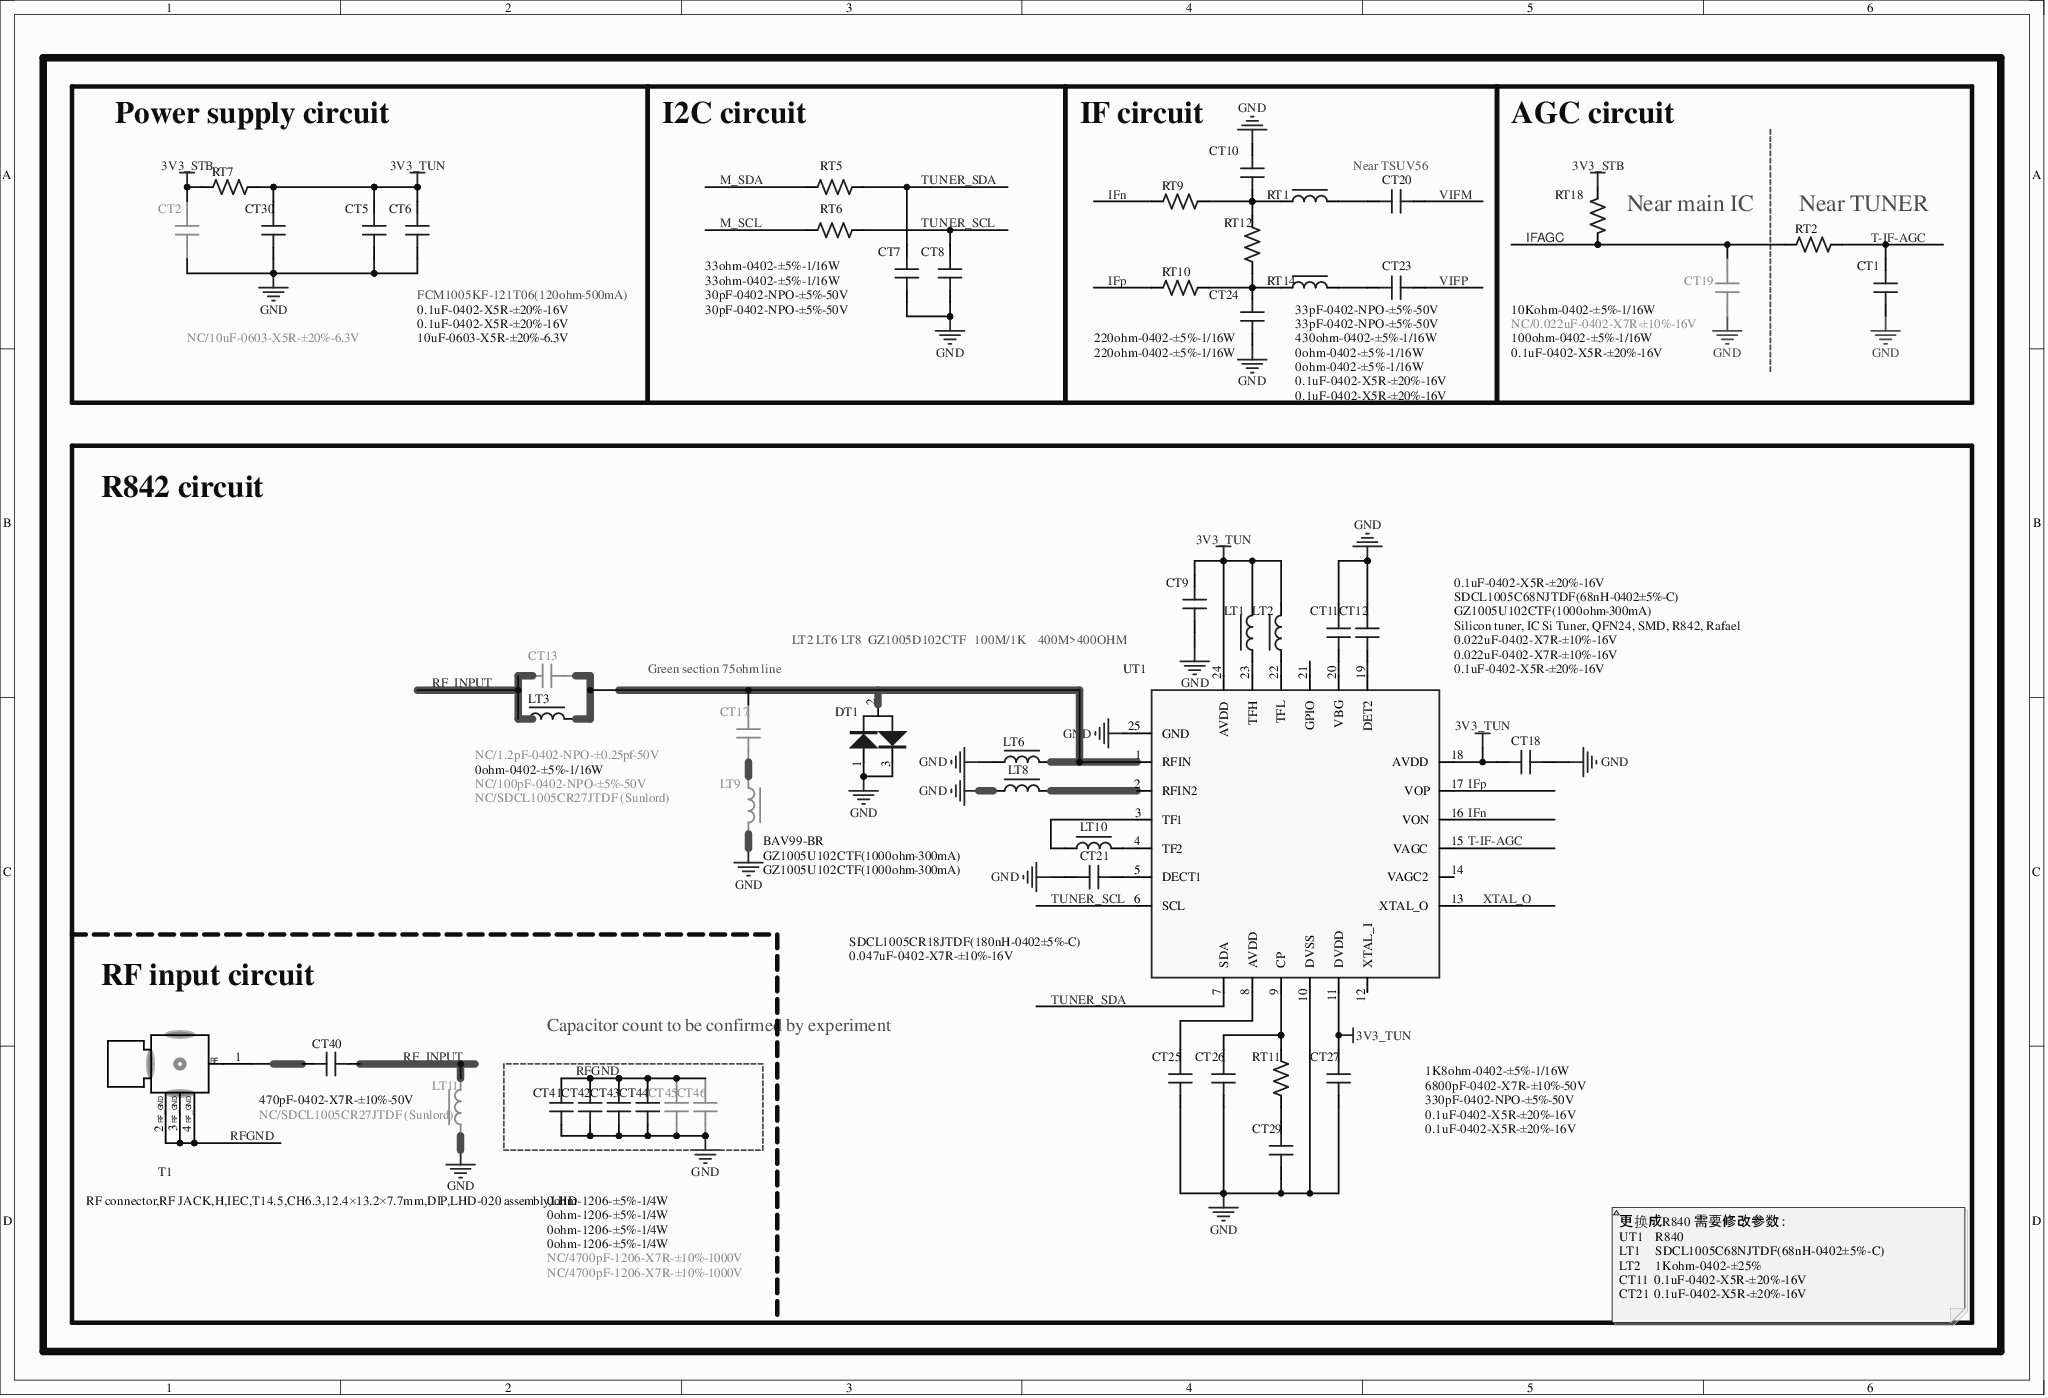
[diagram p0: MISC84277-12.SchDoc]
# Altium project MISC84277-14.PrjPCB (part 10 of 10)

## Sheet MISC84277-12.SchDoc
size 360 x 246 mm

### Parts
CT1  0.1uF-0402-X5R-±20%-16V  [C0402]
CT2  NC/10uF-0603-X5R-±20%-6.3V  [C0603]
CT5  0.1uF-0402-X5R-±20%-16V  [C0402]
CT6  10uF-0603-X5R-±20%-6.3V  [C0603]
CT7  30pF-0402-NPO-±5%-50V  [C0402]
CT8  30pF-0402-NPO-±5%-50V  [C0402]
CT9  0.1uF-0402-X5R-±20%-16V  [C0402]
CT10  33pF-0402-NPO-±5%-50V  [C0402]
CT11  0.022uF-0402-X7R-±10%-16V  [C0402]
CT12  0.022uF-0402-X7R-±10%-16V  [C0402]
CT13  NC/1.2pF-0402-NPO-±0.25pf-50V  [C0402]
CT17  NC/100pF-0402-NPO-±5%-50V  [C0402]
CT18  0.1uF-0402-X5R-±20%-16V  [C0402]
CT19  NC/0.022uF-0402-X7R-±10%-16V  [C0402]
CT20  0.1uF-0402-X5R-±20%-16V  [C0402]
CT21  0.047uF-0402-X7R-±10%-16V  [C0402]
CT23  0.1uF-0402-X5R-±20%-16V  [C0402]
CT24  33pF-0402-NPO-±5%-50V  [C0402]
CT25  0.1uF-0402-X5R-±20%-16V  [C0402]
CT26  330pF-0402-NPO-±5%-50V  [C0402]
CT27  0.1uF-0402-X5R-±20%-16V  [C0402]
CT29  6800pF-0402-X7R-±10%-50V  [C0402]
CT30  0.1uF-0402-X5R-±20%-16V  [C0402]
CT40  470pF-0402-X7R-±10%-50V  [C0402]
CT41  0ohm-1206-±5%-1/4W  [C1206]
CT42  0ohm-1206-±5%-1/4W  [C1206]
CT43  0ohm-1206-±5%-1/4W  [C1206]
CT44  0ohm-1206-±5%-1/4W  [C1206]
CT45  NC/4700pF-1206-X7R-±10%-1000V  [C1206]
CT46  NC/4700pF-1206-X7R-±10%-1000V  [C1206]
DT1  BAV99-BR  [SO-23]
LT1  SDCL1005C68NJTDF(68nH-0402±5%-C)  [L0402]
LT2  GZ1005U102CTF(1000ohm-300mA)  [L0402]
LT3  0ohm-0402-±5%-1/16W  [L0402]
LT6  GZ1005U102CTF(1000ohm-300mA)  [L0402]
LT8  GZ1005U102CTF(1000ohm-300mA)  [L0402]
LT9  NC/SDCL1005CR27JTDF (Sunlord)  [L0402]
LT10  SDCL1005CR18JTDF(180nH-0402±5%-C)  [L0402]
LT11  NC/SDCL1005CR27JTDF (Sunlord)  [L0402]
RT1  0ohm-0402-±5%-1/16W  [L0402]
RT2  100ohm-0402-±5%-1/16W  [R0402]
RT5  33ohm-0402-±5%-1/16W  [R0402]
RT6  33ohm-0402-±5%-1/16W  [R0402]
RT7  FCM1005KF-121T06(120ohm-500mA)  [R0402]
RT9  220ohm-0402-±5%-1/16W  [R0402]
RT10  220ohm-0402-±5%-1/16W  [R0402]
RT11  1K8ohm-0402-±5%-1/16W  [R0402]
RT12  430ohm-0402-±5%-1/16W  [R0402]
RT14  0ohm-0402-±5%-1/16W  [L0402]
RT18  10Kohm-0402-±5%-1/16W  [R0402]
T1  RF connector,RF JACK,H,IEC,T14.5,CH6.3,12.4×13.2×7.7mm,DIP,LHD-020 assembly,LHD  [ANT-IEC14.5-H-短体-NG]
UT1  Silicon tuner, IC Si Tuner, QFN24, SMD, R842, Rafael  [QFN24/0.5-3]

### Blocks framed on the sheet
Power supply circuit: CT2 CT5 CT6 CT30 RT7
I2C circuit: CT7 CT8 RT5 RT6
IF circuit: CT10 CT20 CT23 CT24 RT1 RT9 RT10 RT12 RT14
AGC circuit: CT1 CT19 RT2 RT18

### Nets
3V3_STB: CT2.1 RT7.1 RT18.1
3V3_TUN: CT5.2 CT6.1 CT9.1 CT18.2 CT27.1 CT30.2 LT1.1 LT2.2 RT7.2 UT1.11(DVDD) UT1.18(AVDD) UT1.24(AVDD)
GND: CT1.1 CT2.2 CT5.1 CT6.2 CT7.1 CT8.1 CT9.2 CT10.2 CT11.1 CT12.2 CT18.1 CT19.1 CT21.2 CT24.1 CT25.2 CT26.1 CT27.2 CT29.1 CT30.1 CT41.1 CT42.1 CT43.1 CT44.1 CT45.1 CT46.1 DT1.1 DT1.3 LT6.2 LT8.2 LT9.1 LT11.2 UT1.10(DVSS) UT1.25(GND)
IFAGC: CT19.2 RT2.1 RT18.2
IFn: RT9.2 UT1.16(VON)
IFp: RT10.2 UT1.17(VOP)
M_SCL: RT6.1
M_SDA: RT5.1
RF_INPUT: CT13.1 CT40.2 LT3.1 LT11.1
RFGND: CT41.2 CT42.2 CT43.2 CT44.2 CT45.2 CT46.2 T1.2 T1.3 T1.4
T-IF-AGC: CT1.2 RT2.2 UT1.15(VAGC)
TUNER_SCL: CT8.2 RT6.2 UT1.6(SCL)
TUNER_SDA: CT7.2 RT5.2 UT1.7(SDA)
VIFM: CT20.2
VIFP: CT23.2
XTAL_O: UT1.13(XTAL_O)
NetCT10_1: CT10.1 RT1.1 RT9.1 RT12.2
NetCT11_2: CT11.2 UT1.20(VBG)
NetCT12_1: CT12.1 UT1.19(DET2)
NetCT13_2: CT13.2 CT17.2 DT1.2 LT3.2 LT6.1 UT1.1(RFIN)
NetCT17_1: CT17.1 LT9.2
NetCT20_1: CT20.1 RT1.2
NetCT21_1: CT21.1 UT1.5(DECT1)
NetCT23_1: CT23.1 RT14.2
NetCT24_2: CT24.2 RT10.1 RT12.1 RT14.1
NetCT25_1: CT25.1 UT1.8(AVDD)
NetCT26_2: CT26.2 RT11.2 UT1.9(CP)
NetCT29_2: CT29.2 RT11.1
NetCT40_1: CT40.1 T1.1
NetLT1_2: LT1.2 UT1.23(TFH)
NetLT2_1: LT2.1 UT1.22(TFL)
NetLT8_1: LT8.1 UT1.2(RFIN2)
NetLT10_1: LT10.1 UT1.4(TF2)
NetLT10_2: LT10.2 UT1.3(TF1)

Not connected (* = marked no-connect by the designer): UT1 12(XTAL_I)* 14(VAGC2)* 21(GPIO)*

### Notes on the sheet
- Near TSUV56
- Near main IC
- (near RT2) Near TUNER
- R842 circuit
- (near CT17) Green section 75ohm line
- LT2 LT6 LT8  GZ1005D102CTF   100M/1K    400M>400OHM
- RF input circuit
- Capacitor count to be confirmed by experiment
- 更换成R840 需要修改参数：
  UT1    R840
  LT1      SDCL1005C68NJTDF(68nH-0402±5%-C)
  LT2     1Kohm-0402-±25%
  CT11  0.1uF-0402-X5R-±20%-16V
  CT21  0.1uF-0402-X5R-±20%-16V

### Library data of the parts
CT1 CT5 CT9 CT11 CT18 CT20 CT21 CT23 CT25 CT27 CT30 = 0.1uF-0402-Y5V-+80%-20%-16V-D
CT2 CT6 = 10uF-0603-X5R-±20%-6.3V-D
CT7 CT8 = 33pF-0402-NPO-±5%-50V-D
CT10 CT24 = 56pF-0402-NPO-±5%-50V-D
CT12 CT19 = 0.022uF-0402-X7R-±10%-16V-D
CT13 = 1.8pF-0402-NPO-±0.25pF-50V-D
CT17 = 100pF-0402-NPO-±5%-50V-D
CT26 = 330pF-0402-NPO-±5%-50V-D
CT29 = 6800pF-0402-X7R-±10%-50V-D
CT40 = 470pF-0402-X7R-±10%-50V-D
CT41-CT46 = 1000pF-1206-X7R-±20%-2000V-D
DT1 = BAV99-BR-D
LT1 = SDCL1005C68NJTDF(68nH-0402±5%-C)-D
LT2 LT6 LT8 RT1 RT14 = 1Kohm-0402-±25%-D
LT3 = 2.2nH-0402-±0.3nH-1/4-D
LT9 LT11 = SDCL1005CR27JTDF(顺络)-D
LT10 = SDCL1608CR22JT(F)-D
RT2 = 100ohm-0402-±5%-1/16W-D
RT5 RT6 = 33ohm-0402-±5%-1/16W-D
RT7 = 0ohm-0402-±5%-1/16W-D
RT9 RT10 = 220ohm-0402-±5%-1/16W-D
RT11 = 1K8ohm-0402-±5%-1/16W-D
RT12 = 820ohm-0402-±5%-1/16W-D
RT18 = 10Kohm-0402-±5%-1/16W-D
T1 = RF-A814.5(H=6.3mm)-DLMI: T-IEC-6.3mm-#-#
UT1 = R840-D

## Nets that join several sheets
1.15V_STB: MISC84277-7 (7 pins), MISC84277-8 (13 pins)
3V3_STB: MISC84277-7 (6 pins), PCBE84277 (RB354.2), MISC84277-8 (24 pins), MISC84277-12 (CT2.1 RT7.1 RT18.1)
5V_M: MISC84277-7 (CL42.1 CM2.1 QM1.D UL1.2), PCBE84277 (DB901.1 DB901.3 RB346.1), MISC84277-8 (RK2.2), MISC84277-9 (F2.1), MISC84277-10 (AVH2.18 AVH3.18)
5V_STB: MISC84277-7 (16 pins), PCBE84277 (RB301.2 RB384.1), MISC84277-8 (RF8.2 RF9.2 RK1.1 RK15.1)
12V: MISC84277-7 (7 pins), PCBE84277 (11 pins), MISC84277-11 (10 pins)
+1.8V_DDR: MISC84277-7 (5 pins), MISC84277-8 (7 pins)
BL_ON: MISC84277-7 (CG1.1 RG1.1), PCBE84277 (BL_ON.1 RB386.2)
GND: MISC84277-3 (28 pins), MISC84277-7 (36 pins), PCBE84277 (44 pins), MISC84277-8 (58 pins), MISC84277-9 (67 pins), MISC84277-10 (49 pins), MISC84277-11 (22 pins), MISC84277-12 (33 pins)
PWM_REF: MISC84277-7 (CG2.1 RG2.2), PCBE84277 (PWM_REF.1 RB366.2)
VCC_PANEL: MISC84277-7 (CM4.1 CM7.1 QM5.D RM6.1), MISC84277-8 (CN12.1 CN12.2 CN12.3)
AMP-OUTL: MISC84277-8 (CF29.1 RF14.2 U1.41), MISC84277-11 (RA4.1)
AMP-OUTR: MISC84277-8 (CF30.1 RF15.2 U1.42), MISC84277-11 (RA12.1)
AMP_STB: MISC84277-8 (U1.81), MISC84277-11 (RA1.2 RA8.1)
AV1_LIN: MISC84277-8 (U1.32), MISC84277-9 (CI3.1)
AV1_RIN: MISC84277-8 (U1.31), MISC84277-9 (CI4.1)
AV2_LIN: MISC84277-8 (U1.36), MISC84277-9 (CI5.1)
AV2_RIN: MISC84277-8 (U1.35), MISC84277-9 (CI6.1)
AV-OUTL: MISC84277-8 (U1.39), MISC84277-9 (RO5.1)
AV-OUTR: MISC84277-8 (U1.40), MISC84277-9 (RO1.1)
AV_IN: MISC84277-8 (U1.27), MISC84277-9 (CI1.1)
CVBS_OUT: MISC84277-8 (U1.29), MISC84277-9 (CO9.2 RO2.2 RO12.1 RO13.2)
DDC_SCL: MISC84277-8 (RF11.2), MISC84277-9 (CN11.15)
DDC_SDA: MISC84277-8 (RF10.2), MISC84277-9 (CN11.12)
HDMI1_HPDIN: MISC84277-8 (U1.113), MISC84277-10 (RH15.2 RH16.2)
HDMI1_RX0_N: MISC84277-8 (U1.1), MISC84277-10 (CN14.9 UH3.3 UH3.6)
HDMI1_RX0_P: MISC84277-8 (U1.2), MISC84277-10 (CN14.7 UH3.4 UH3.5)
HDMI1_RX1_N: MISC84277-8 (U1.3), MISC84277-10 (CN14.6 UH1.1 UH1.8)
HDMI1_RX1_P: MISC84277-8 (U1.4), MISC84277-10 (CN14.4 UH1.2 UH1.7)
HDMI1_RX2_N: MISC84277-8 (U1.5), MISC84277-10 (CN14.3 UH1.3 UH1.6)
HDMI1_RX2_P: MISC84277-8 (U1.6), MISC84277-10 (CN14.1 UH1.4 UH1.5)
HDMI1_RXC_N: MISC84277-8 (U1.127), MISC84277-10 (CN14.12 UH3.1 UH3.8)
HDMI1_RXC_P: MISC84277-8 (U1.128), MISC84277-10 (CN14.10 UH3.2 UH3.7)
HDMI1_SCL: MISC84277-8 (U1.108), MISC84277-10 (RH10.1)
HDMI1_SDA: MISC84277-8 (U1.107), MISC84277-10 (RH11.1)
HDMI3_CLKN: MISC84277-8 (U1.119), MISC84277-10 (5 pins)
HDMI3_CLKP: MISC84277-8 (U1.120), MISC84277-10 (5 pins)
HDMI3_HPDIN: MISC84277-8 (U1.112), MISC84277-10 (RH6.2 RH7.2)
HDMI3_RX0N: MISC84277-8 (U1.121), MISC84277-10 (5 pins)
HDMI3_RX0P: MISC84277-8 (U1.122), MISC84277-10 (5 pins)
HDMI3_RX1N: MISC84277-8 (U1.123), MISC84277-10 (5 pins)
HDMI3_RX1P: MISC84277-8 (U1.124), MISC84277-10 (5 pins)
HDMI3_RX2N: MISC84277-8 (U1.125), MISC84277-10 (5 pins)
HDMI3_RX2P: MISC84277-8 (U1.126), MISC84277-10 (5 pins)
HDMI3_SCL: MISC84277-8 (U1.99), MISC84277-10 (RH3.1)
HDMI3_SDA: MISC84277-8 (U1.98), MISC84277-10 (RH4.1)
HDMI_ARC: MISC84277-8 (U1.117), MISC84277-10 (CH15.1)
HDMI_CEC: MISC84277-8 (U1.111), MISC84277-10 (RH13.1)
HDMI_DET: MISC84277-8 (U1.102), MISC84277-10 (RH55.1 RH56.1)
IFAGC: MISC84277-8 (U1.43), MISC84277-12 (CT19.2 RT2.1 RT18.2)
M_SCL: MISC84277-8 (RT3.2 U1.52), MISC84277-10 (RH19.1), MISC84277-12 (RT6.1)
M_SDA: MISC84277-8 (RT4.2 U1.51), MISC84277-10 (RH20.1), MISC84277-12 (RT5.1)
PC_LIN: MISC84277-8 (U1.38), MISC84277-9 (CV6.2)
PC_RIN: MISC84277-8 (U1.37), MISC84277-9 (CV5.2)
PWM0: MISC84277-7 (RG2.1), MISC84277-8 (RF13.1 U1.86)
PWM1: MISC84277-7 (RG1.2), MISC84277-8 (RF18.1 U1.87)
PWR_ON/OFF: MISC84277-7 (RM3.2 RM4.2 RM8.1), MISC84277-8 (U1.84)
SPDIF_OUT: MISC84277-8 (U1.85), MISC84277-9 (CO8.1 RO9.1)
USB0_DM: MISC84277-8 (U1.59), MISC84277-9 (RU1.1)
USB0_DP: MISC84277-8 (U1.60), MISC84277-9 (RU3.1)
USB1_DM: MISC84277-8 (U1.57), MISC84277-9 (RU2.1)
USB1_DP: MISC84277-8 (U1.58), MISC84277-9 (RU4.1)
VGA_BIN: MISC84277-8 (U1.17), MISC84277-9 (CV7.1)
VGA_GIN: MISC84277-8 (U1.18), MISC84277-9 (CV3.1)
VGA_HS: MISC84277-8 (U1.16), MISC84277-9 (CV9.1 RV12.2)
VGA_RIN: MISC84277-8 (U1.20), MISC84277-9 (CV1.1)
VGA_VS: MISC84277-8 (U1.21), MISC84277-9 (CV10.1 RV10.2)
VIFM: MISC84277-8 (U1.45), MISC84277-12 (CT20.2)
VIFP: MISC84277-8 (U1.44), MISC84277-12 (CT23.2)
XTAL_O: MISC84277-8 (LF7.2), MISC84277-12 (UT1.13)
YPBPR_PB: MISC84277-8 (U1.23), MISC84277-9 (CI9.1)
YPBPR_PR: MISC84277-8 (U1.26), MISC84277-9 (CI11.1)
YPBPR_Y: MISC84277-8 (U1.24), MISC84277-9 (CI7.1)